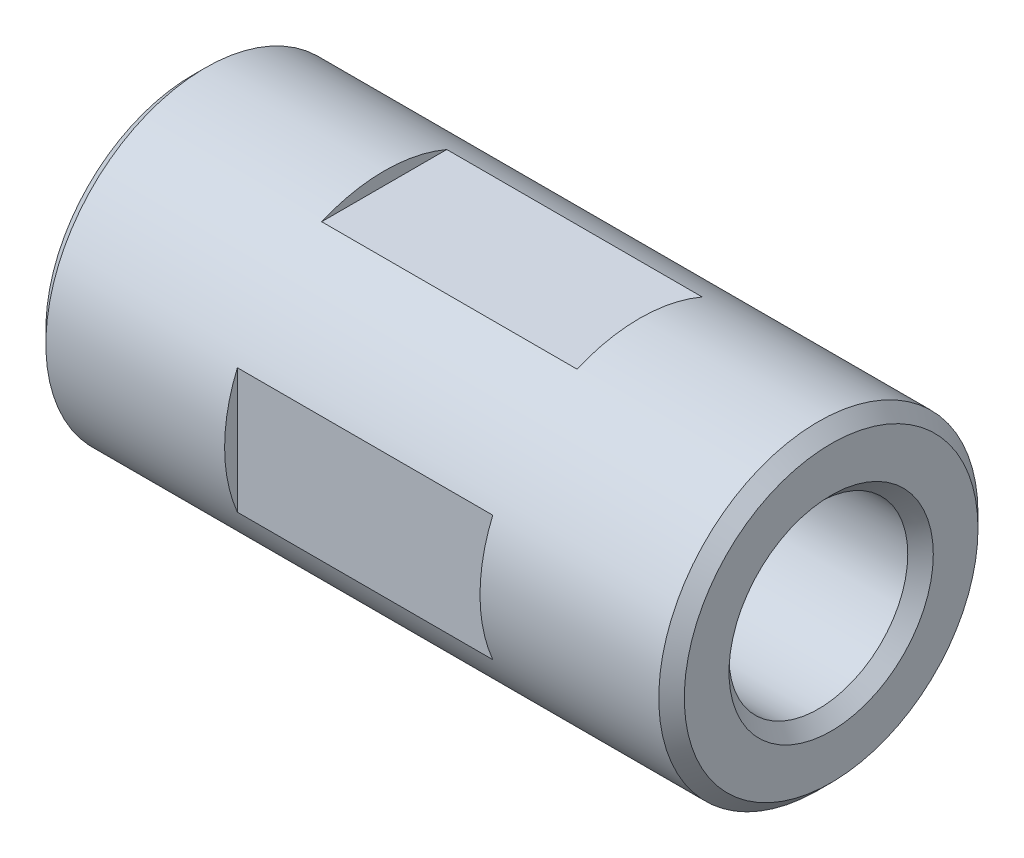
SolidWorks part; units mm, degrees
ref_plane "前视基准面" through (0, 0, 0) normal (0, 0, 1) x (1, 0, 0)
ref_plane "上视基准面" through (0, 0, 0) normal (0, 1, 0) x (1, 0, 0)
ref_plane "右视基准面" through (0, 0, 0) normal (1, 0, 0) x (0, 0, -1)
sketch "草图1" plane through (0, 0, 0) normal (1, 0, 0) x (0, 0, -1)
  circle A0 centre (0, 0) radius 12.5
  dimension "D1" = 25
extrude "凸台-拉伸1" add sketch "草图1" along normal mid plane 50
hole_wizard "M16 螺纹孔1" positions "草图2" profile "草图3" tap size "M16" standard "GB" end condition through all
sketch "草图2" plane through (25, 0, 0) normal (1, 0, 0) x (0, 0, -1)
  point P0 (0, 0)
sketch "草图3" plane through (25, 0, 0) normal (0, 1, 0) x (0, 0, -1)
  line L0 (0, 0) -> (0, 50)
  line L1 (0, 50) -> (7, 50)
  line L2 (7, 50) -> (7, 0)
  line L5 (7, 0) -> (0, 0)
  line L11 (0, -6.35) -> (0, 107.95) construction
  dimension "通孔螺纹孔钻头直径" = 14
  dimension "通孔螺纹孔钻头深度" = 50
cosmetic thread "孔螺蚊线1" parameters "D2"=16
sketch "草图4" plane through (0, 0, 0) normal (1, 0, 0) x (0, 0, -1)
  line L1 (-11.5, 11.5) -> (11.5, 11.5)
  line L2 (-11.5, 11.5) -> (-11.5, -11.5)
  line L3 (-11.5, -11.5) -> (11.5, -11.5)
  line L4 (11.5, 11.5) -> (11.5, -11.5)
  line L5 (-11.5, 11.5) -> (11.5, -11.5) construction
  line L6 (-11.5, -11.5) -> (11.5, 11.5) construction
  point P0 (0, 0)
  dimension "D1" = 23
extrude "切除-拉伸1" cut sketch "草图4" against normal mid plane 20 flip side to cut
chamfer "倒角1" distance 1 angle 45 4 edges at (-25, 0, -7) (25, 0, -7) (25, 0, -12.5) (-25, 0, -12.5)
